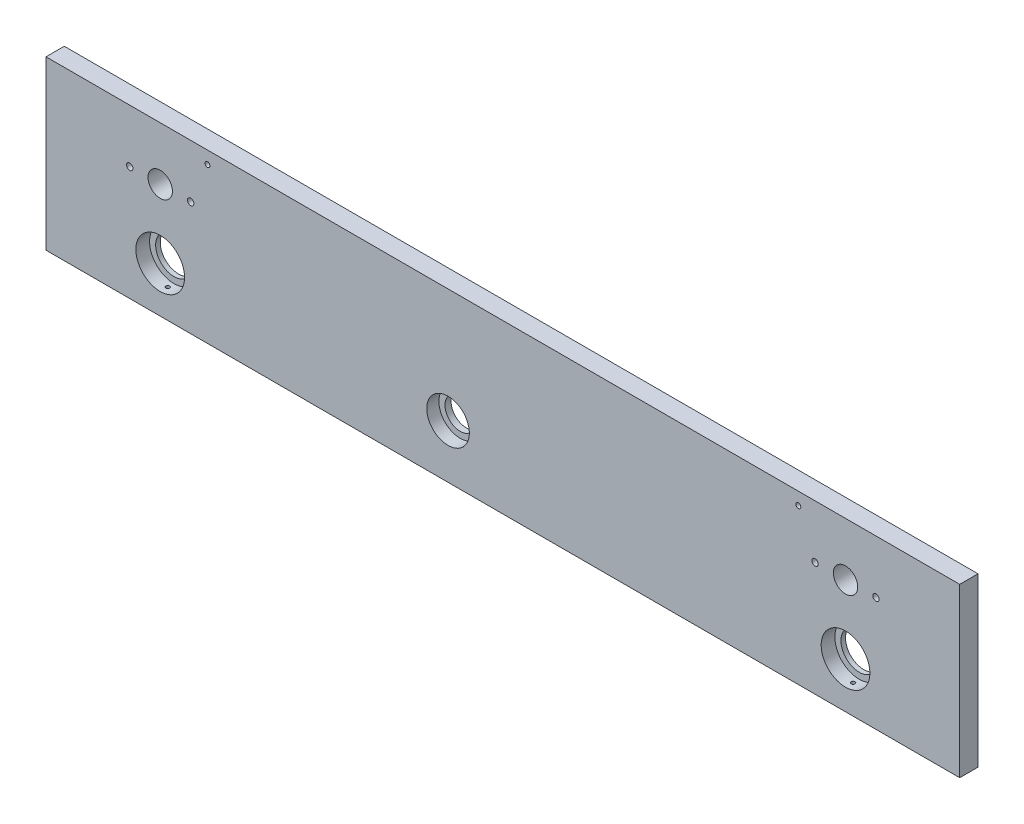
SolidWorks part; units mm, degrees
ref_plane "前视基准面" through (0, 0, 0) normal (0, 0, 1) x (1, 0, 0)
ref_plane "上视基准面" through (0, 0, 0) normal (0, 1, 0) x (1, 0, 0)
ref_plane "右视基准面" through (0, 0, 0) normal (1, 0, 0) x (0, 0, -1)
sketch "草图1" plane through (0, 0, 0) normal (0, 0, 1) x (1, 0, 0)
  line L0 (-300, -30) -> (-300, 0)
  line L1 (-300, 0) -> (300, 0)
  line L2 (300, -30) -> (300, 0)
  line L3 (0, 17.0098) -> (0, -58.9914) construction
  line L4 (-300, -110) -> (300, -110)
  line L7 (-300, -30) -> (-300, -110)
  line L10 (300, -30) -> (300, -110)
  point P0 (0, 0)
  point P1 (0, 0)
  point P10 (0, -110)
  point P14 (0, -130)
  dimension "D1" = 110
  dimension "D2" = 600
  dimension "D3" = 80
extrude "凸台-拉伸1" add sketch "草图1" along normal blind 12
sketch "草图2" plane through (0, 0, 12) normal (0, 0, 1) x (1, 0, 0)
  line L0 (-300, -110) -> (300, -110) construction
  line L3 (0, 56.4345) -> (0, -12.8032) construction
  line L4 (-300, 0) -> (-300, -110) construction
  circle A0 centre (225, -80) radius 16
  circle A3 centre (-225, -80) radius 16
  dimension "D1" = 32
  dimension "D2" = 30
  dimension "D5" = 75
extrude "切除-拉伸2" cut sketch "草图2" against normal blind 9
sketch "草图3" plane through (0, 0, 12) normal (0, 0, 1) x (1, 0, 0)
  line L0 (-300, -110) -> (300, -110) construction
  line L1 (-300, 0) -> (-300, -110) construction
  circle A0 centre (-36, -75) radius 14
  dimension "D1" = 28
  dimension "D2" = 35
  dimension "D3" = 264
extrude "切除-拉伸3" cut sketch "草图3" against normal blind 8
sketch "草图4" plane through (0, 0, 4) normal (0, 0, 1) x (1, 0, 0)
  circle A0 centre (-36, -75) radius 10
  dimension "D1" = 20
extrude "切除-拉伸4" cut sketch "草图4" against normal through all
hole_wizard "M4 螺纹孔2" positions "草图10" profile "草图9" tap size "M4" standard "Iso" end condition through all
sketch "草图10" plane through (0, 0, 0) normal (0, 0, -1) x (-1, 0, 0)
  point P0 (-194, -8.25)
  point P2 (194, -8.25)
sketch "草图9" plane through (194, -8.25, 0) normal (1, 0, 0) x (0, 1, 0)
  line L0 (0, 0) -> (0, 12)
  line L1 (0, 12) -> (1.65, 12)
  line L2 (1.65, 12) -> (1.65, 0)
  line L5 (1.65, 0) -> (0, 0)
  line L11 (0, -6.35) -> (0, 107.95) construction
  dimension "通孔螺纹孔钻头直径" = 3.3
  dimension "通孔螺纹孔钻头深度" = 12
cosmetic thread "孔螺蚊线7" parameters "D2"=4
cosmetic thread "孔螺蚊线8" parameters "D2"=4
hole_wizard "M4 螺纹孔3" positions "草图12" profile "草图11" tap size "M4" standard "Iso"
sketch "草图12" plane through (0, -110, 0) normal (0, -1, 0) x (-1, 0, 0)
  line L0 (300, 0) -> (-300, 0) construction
  line L1 (300, -12) -> (300, 0) construction
  line L2 (-300, -12) -> (-300, 0) construction
  point P0 (-262, -6)
  point P2 (-92, -6)
  point P4 (92, -6)
  point P6 (262, -6)
  dimension "D1" = 6
  dimension "D2" = 38
  dimension "D3" = 170
  dimension "D4" = 38
  dimension "D5" = 170
sketch "草图11" plane through (262, -110, 6) normal (1, 0, 0) x (0, 0, -1)
  line L0 (0, 0) -> (0, 13.0914)
  line L1 (0, 13.0914) -> (1.65, 12.1)
  line L2 (1.65, 12.1) -> (1.65, 0)
  line L5 (1.65, 0) -> (0, 0)
  line L10 (0, 13.0914) -> (-1.65, 12.1) construction
  line L11 (0, -6.35) -> (0, 107.95) construction
  dimension "螺纹孔钻头直径" = 3.3
  dimension "螺纹孔钻头深度" = 12.1
  dimension "导头角度" = 118
cosmetic thread "孔螺蚊线9" parameters "D1"=10, "D2"=4
cosmetic thread "孔螺蚊线10" parameters "D1"=10, "D2"=4
cosmetic thread "孔螺蚊线11" parameters "D1"=10, "D2"=4
cosmetic thread "孔螺蚊线12" parameters "D1"=10, "D2"=4
hole_wizard "M3 螺纹孔1" positions "草图16" profile "草图15" tap size "M3" standard "Iso"
sketch "草图16" plane through (0, -110, 0) normal (0, -1, 0) x (-1, 0, 0)
  line L0 (300, 0) -> (-300, 0) construction
  line L1 (300, -12) -> (300, 0) construction
  line L2 (-300, -12) -> (-300, 0) construction
  point P0 (225, -7)
  point P2 (-225, -7)
  dimension "D1" = 7
  dimension "D2" = 7
  dimension "D3" = 75
  dimension "D4" = 75
sketch "草图15" plane through (-225, -110, 7) normal (1, 0, 0) x (0, 0, -1)
  line L0 (0, 0) -> (0, 14)
  line L1 (0, 14) -> (1.25, 14)
  line L2 (1.25, 14) -> (1.25, 0)
  line L5 (1.25, 0) -> (0, 0)
  line L11 (0, -6.35) -> (0, 107.95) construction
  dimension "通孔螺纹孔钻头直径" = 2.5
  dimension "通孔螺纹孔钻头深度" = 14
cosmetic thread "孔螺蚊线13" parameters "D2"=3
cosmetic thread "孔螺蚊线14" parameters "D2"=3
sketch "草图17" plane through (0, 0, 3) normal (0, 0, 1) x (1, 0, 0)
  circle A0 centre (-225, -80) radius 12
  circle A1 centre (225, -80) radius 12
  dimension "D1" = 24
  dimension "D2" = 24
extrude "切除-拉伸5" cut sketch "草图17" against normal through all
sketch "草图18" plane through (0, 0, 12) normal (0, 0, 1) x (1, 0, 0)
  line L0 (-300, 0) -> (-300, -110) construction
  line L1 (300, 0) -> (-300, 0) construction
  line L2 (0, 53.9596) -> (0, -25.2282) construction
  circle A0 centre (-225, -35) radius 8
  circle A1 centre (225, -35) radius 8
  dimension "D3" = 16
  dimension "D1" = 75
  dimension "D2" = 35
extrude "切除-拉伸6" cut sketch "草图18" against normal through all
hole_wizard "M5 螺纹孔1" positions "草图21" profile "草图20" tap size "M5" standard "Iso" end condition through all
sketch "草图21" plane through (0, 0, 12) normal (0, 0, 1) x (1, 0, 0)
  point P0 (245, -35)
  point P3 (205, -35)
  point P6 (-245, -35)
  point P9 (-205, -35)
sketch "草图20" plane through (245, -35, 12) normal (1, 0, 0) x (0, -1, 0)
  line L0 (0, 0) -> (0, 12)
  line L1 (0, 12) -> (2.1, 12)
  line L2 (2.1, 12) -> (2.1, 0)
  line L5 (2.1, 0) -> (0, 0)
  line L11 (0, -6.35) -> (0, 107.95) construction
  dimension "通孔螺纹孔钻头直径" = 4.2
  dimension "通孔螺纹孔钻头深度" = 12
cosmetic thread "孔螺蚊线15" parameters "D2"=5
cosmetic thread "孔螺蚊线16" parameters "D2"=5
cosmetic thread "孔螺蚊线17" parameters "D2"=5
cosmetic thread "孔螺蚊线18" parameters "D2"=5
